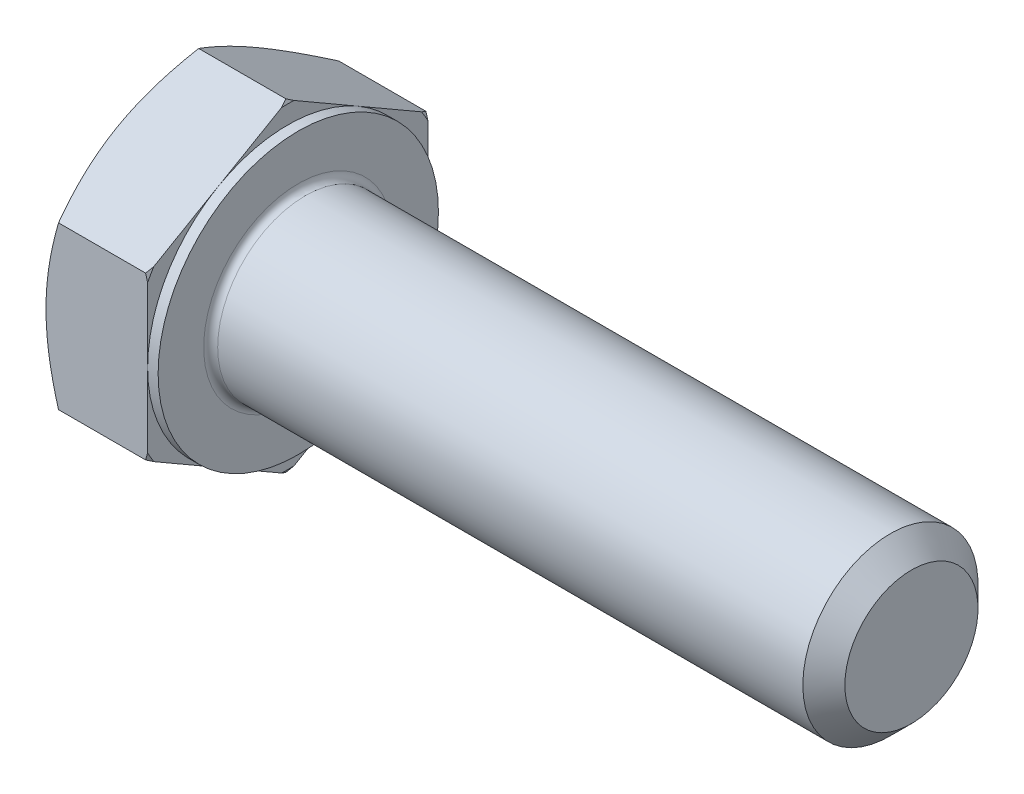
from build123d import *

# Parameters (mm, degrees)
EXTRUDE_368_DEPTH = 6.4
SKETCH_4_W        = 0.6
SKETCH_4_H        = 11.237604307
CHAMFER_1891_SIZE = 1.2
FILLET_1936_R     = 0.4


with BuildPart() as part:
    # 草图1 → Extrude 368 (new body)
    with BuildSketch(Plane(origin=(0, 0, 0), x_dir=(0, 0, -1), z_dir=(1, 0, 0))):
        Polygon((8, 4.618802154), (8, -4.618802154), (0, -9.237604307), (-8, -4.618802154), (-8, 4.618802154), (0, 9.237604307), align=None)
    extrude(amount=EXTRUDE_368_DEPTH)

    # 草图2 → 凸台-旋转1 (revolve)
    with BuildSketch(Plane.XY, mode=Mode.PRIVATE) as revolve_1_sk:
        Polygon((0, 0), (41.4, 0), (41.4, 3.701), (41.4, 5), (0, 5), align=None)
    revolve(revolve_1_sk.sketch.rotate(Axis((0, 0, 0), (1, 0, 0)), 90), axis=Axis((0, 0, 0), (1, 0, 0)))

    # 草图3 → 切除-旋转1 (revolve, cut)
    with BuildSketch(Plane.XY):
        Polygon((0, 8), (3.601282526, 14.237604307), (3.601282526, 19.237604307), (-10, 19.237604307), (-10, 8), align=None)
    revolve(axis=Axis((0, 0, 0), (1, 0, 0)), mode=Mode.SUBTRACT)

    # 草图5 → 切除-旋转2 (revolve, cut)
    with BuildSketch(Plane.XY):
        Polygon((6.4, 8), (2.798717474, 14.237604307), (2.798717474, 19.237604307), (12.798717474, 19.237604307), (12.798717474, 8), align=None)
    revolve(axis=Axis((0, 0, 0), (1, 0, 0)), mode=Mode.SUBTRACT)

    # 草图4 → 切除-旋转3 (revolve, cut)
    with BuildSketch(Plane.XY, mode=Mode.PRIVATE) as cut_revolve_3_sk:
        with Locations((6.1, 13.618802154)):
            Rectangle(SKETCH_4_W, SKETCH_4_H)
    revolve(cut_revolve_3_sk.sketch.rotate(Axis((0, 0, 0), (1, 0, 0)), 270), axis=Axis((0, 0, 0), (1, 0, 0)), mode=Mode.SUBTRACT)

    # Chamfer 1891
    chamfer_1891_edges = [part.edges().sort_by_distance(p)[0] for p in [
        (41.4, 0, -5),
    ]]
    chamfer(chamfer_1891_edges, length=CHAMFER_1891_SIZE)

    # Fillet 1936
    fillet_1936_edges = [part.edges().sort_by_distance(p)[0] for p in [
        (6.4, 0, -5),
    ]]
    fillet(fillet_1936_edges, radius=FILLET_1936_R)


solid = part.part
